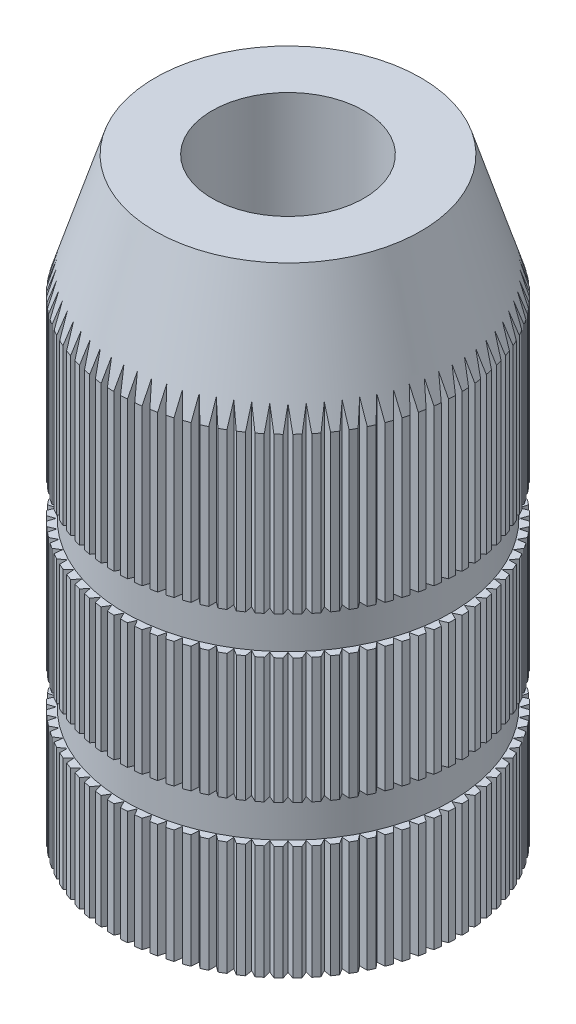
from build123d import *

# Parameters (mm, degrees)
CUT_EXTRUDE_1_DEPTH      = 10
PATTERN_CIRCULAR_1_COUNT = 80
SKETCH_3_W               = 0.303777404
SKETCH_3_H               = 0.5


with BuildPart() as part:
    # 草图1 → 旋转1 (revolve)
    with BuildSketch(Plane.XY, mode=Mode.PRIVATE) as revolve_1_sk:
        Polygon((-2.25, 0), (-2.25, 6.2), (-1.75, 7.8), (-1, 7.8), (-1, 0.2), (-1.2, 0), align=None)
    revolve(revolve_1_sk.sketch.rotate(Axis((0, 0, 0), (0, 1, 0)), 270), axis=Axis((0, 0, 0), (0, 1, 0)))

    # 草图2 → 切除-拉伸1 (cut)
    with BuildSketch(Plane.XZ):
        Polygon((-2.26, 0.05), (-2.26, -0.05), (-2.16, 0), align=None)
    cut_extrude_1 = extrude(amount=-CUT_EXTRUDE_1_DEPTH, mode=Mode.SUBTRACT)

    # 阵列(圆周)1: 切除-拉伸1 ×80 about axis
    pattern_circular_1_axis = Axis((0, 0, 0), (0, 1, 0))
    for i in range(1, PATTERN_CIRCULAR_1_COUNT):
        add(cut_extrude_1.rotate(pattern_circular_1_axis, i * 360 / PATTERN_CIRCULAR_1_COUNT), mode=Mode.SUBTRACT)

    # 草图3 → 切除-旋转1 (revolve, cut)
    with BuildSketch(Plane.XY, mode=Mode.PRIVATE) as cut_revolve_1_sk:
        with Locations((-2.301888702, 1.75)):
            Rectangle(SKETCH_3_W, SKETCH_3_H)
        with Locations((-2.301888702, 3.9)):
            Rectangle(SKETCH_3_W, SKETCH_3_H)
    revolve(cut_revolve_1_sk.sketch.rotate(Axis((0, 0, 0), (0, 1, 0)), 270), axis=Axis((0, 0, 0), (0, 1, 0)), mode=Mode.SUBTRACT)


solid = part.part
